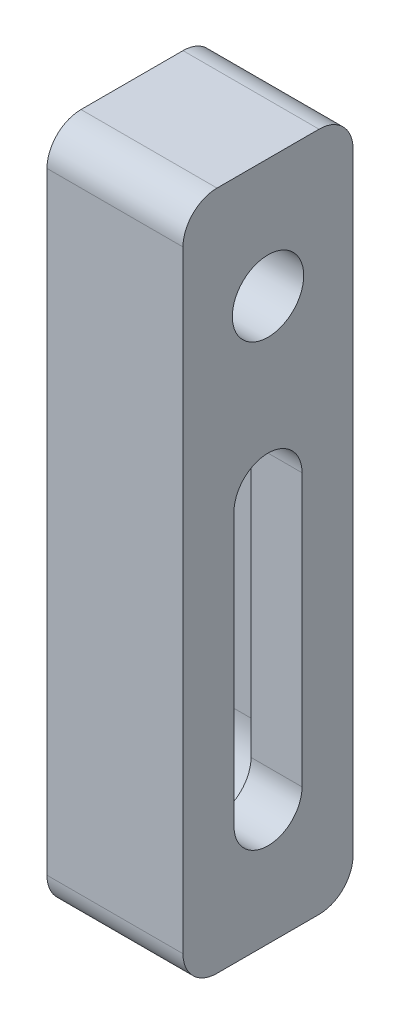
SolidWorks part; units mm, degrees
ref_plane "前视基准面" through (0, 0, 0) normal (0, 0, 1) x (1, 0, 0)
ref_plane "上视基准面" through (0, 0, 0) normal (0, 1, 0) x (1, 0, 0)
ref_plane "右视基准面" through (0, 0, 0) normal (1, 0, 0) x (0, 0, -1)
sketch "草图1" plane through (0, 0, 0) normal (0, 0, 1) x (1, 0, 0)
  line L0 (-9.756, 48.5236) -> (-9.756, 8.5236)
  line L1 (-1.756, 48.5236) -> (-1.756, 8.5236)
  line L2 (-1.756, 8.5236) -> (-9.756, 8.5236)
  line L9 (-9.756, 48.5236) -> (-1.756, 48.5236)
  point P0 (0, 0)
  dimension "D1" = 8
  dimension "D2" = 40
extrude "凸台-拉伸1" add sketch "草图1" along normal blind 10
hole_wizard "M5 螺纹孔1" positions "草图4" profile "草图3" tap size "M5" standard "Iso"
sketch "草图4" plane through (-1.756, 0, 0) normal (1, 0, 0) x (0, 0, -1)
  line L0 (-10, 48.5236) -> (0, 48.5236) construction
  point P0 (-5, 41.5236)
  dimension "D1" = 7
sketch "草图3" plane through (-1.756, 41.5236, 5) normal (0, 1, 0) x (0, 0, -1)
  line L0 (0, 0) -> (0, 13.6618)
  line L1 (0, 13.6618) -> (2.1, 12.4)
  line L2 (2.1, 12.4) -> (2.1, 0)
  line L5 (2.1, 0) -> (0, 0)
  line L10 (0, 13.6618) -> (-2.1, 12.4) construction
  line L11 (0, -6.35) -> (0, 107.95) construction
  dimension "螺纹孔钻头直径" = 4.2
  dimension "螺纹孔钻头深度" = 12.4
  dimension "导头角度" = 118
cosmetic thread "孔螺蚊线1" parameters "D1"=8, "D2"=5
fillet "圆角1" radius 2 2 edges at (-5.756, 48.5236, 0) (-5.756, 48.5236, 10)
sketch "草图5" plane through (-9.756, 0, 0) normal (-1, 0, 0) x (0, 0, 1)
  line L0 (5, 15.5236) -> (5, 31.5236) construction
  line L1 (3, 15.5236) -> (3, 31.5236)
  line L2 (7, 15.5236) -> (7, 31.5236)
  line L3 (10, 8.5236) -> (0, 8.5236) construction
  arc A0 (3, 15.5236) -> (7, 15.5236) centre (5, 15.5236) ccw
  arc A1 (7, 31.5236) -> (3, 31.5236) centre (5, 31.5236) ccw
  point P2 (5, 23.5236)
  point P9 (5, 8.5236)
  dimension "D2" = 2
  dimension "D1" = 16
  dimension "D3" = 7
extrude "切除-拉伸1" cut sketch "草图5" against normal through all
sketch "草图6" plane through (-9.756, 0, 0) normal (-1, 0, 0) x (0, 0, 1)
  line L0 (5, 31.5236) -> (5, 15.5236) construction
  line L1 (9, 31.5236) -> (9, 15.5236)
  line L2 (1, 31.5236) -> (1, 15.5236)
  arc A0 (9, 31.5236) -> (1, 31.5236) centre (5, 31.5236) ccw
  arc A1 (1, 15.5236) -> (9, 15.5236) centre (5, 15.5236) ccw
  point P4 (5, 23.5236)
  dimension "D1" = 4
extrude "切除-拉伸2" cut sketch "草图6" against normal blind 5
fillet "圆角2" radius 2 2 edges at (-5.756, 8.5236, 0) (-5.756, 8.5236, 10)
